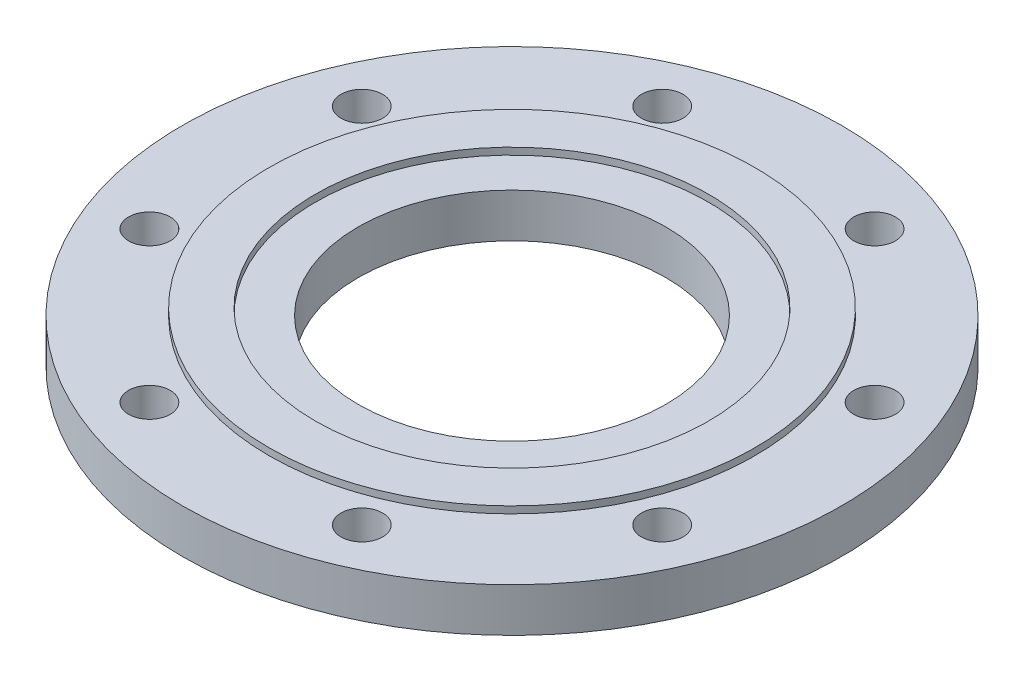
SolidWorks part; units mm, degrees
material "AISI 304"
ref_plane "Front Plane" through (0, 0, 0) normal (0, 0, 1) x (1, 0, 0)
ref_plane "Top Plane" through (0, 0, 0) normal (0, 1, 0) x (1, 0, 0)
ref_plane "Right Plane" through (0, 0, 0) normal (1, 0, 0) x (0, 0, -1)
sketch "Sketch1" plane through (0, 0, 0) normal (0, 1, 0) x (1, 0, 0)
  circle A0 centre (0, 0) radius 142.5
  circle A1 centre (0, 0) radius 66.5
  dimension "D1" = 285
  dimension "D2" = 133
extrude "Boss-Extrude1" add sketch "Sketch1" along normal mid plane 19
sketch "Sketch2" plane through (0, 9.5, 0) normal (0, 1, 0) x (1, 0, 0)
  circle A0 centre (0, 0) radius 85
  circle A1 centre (0, 0) radius 105
  dimension "D1" = 170
  dimension "D2" = 210
extrude "Boss-Extrude2" add sketch "Sketch2" along normal blind 3
sketch "Sketch3" plane through (0, 9.5, 0) normal (0, 1, 0) x (1, 0, 0)
  line L0 (0, 0) -> (-45.922, 110.8655) construction
  line L1 (0, 0) -> (0, 120) construction
  circle A0 centre (0, 0) radius 120 construction
  circle A1 centre (-45.922, 110.8655) radius 9
  dimension "D1" = 240
  dimension "D3" = 18
  dimension "D2" = 22.5
extrude "Cut-Extrude1" cut sketch "Sketch3" against normal through all
pattern_circular "CirPattern1" count 8 over 360 about axis through (0, 0, 0) along (0, 1, 0) of "Cut-Extrude1"
